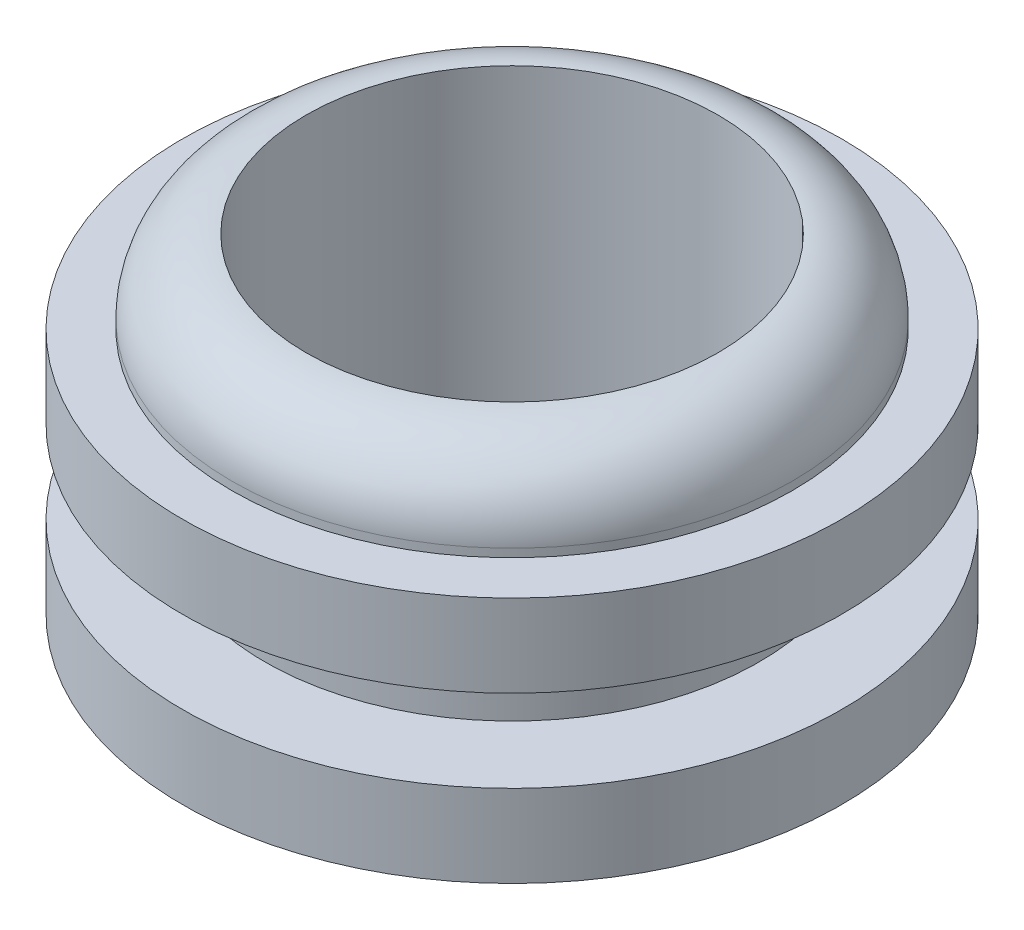
from build123d import *


with BuildPart() as part:
    # 草图1 → 旋转1 (revolve)
    with BuildSketch(Plane.XY, mode=Mode.PRIVATE) as revolve_1_sk:
        with BuildLine():
            Line((2.5, 0), (4, 0))
            Line((4, 0), (4, 1))
            Line((4, 1), (3, 1))
            Line((3, 1), (3, 2))
            Line((3, 2), (4, 2))
            Line((4, 2), (4, 3))
            Line((4, 3), (3.4, 3))
            Line((3.4, 3), (3.4, 3.1))
            ThreePointArc((3.4, 3.1), (3.136396103, 3.736396103), (2.5, 4))
            Line((2.5, 4), (2.5, 0))
        make_face()
    revolve(revolve_1_sk.sketch.rotate(Axis((0, 0, 0), (0, 1, 0)), 90), axis=Axis((0, 0, 0), (0, 1, 0)))


solid = part.part
